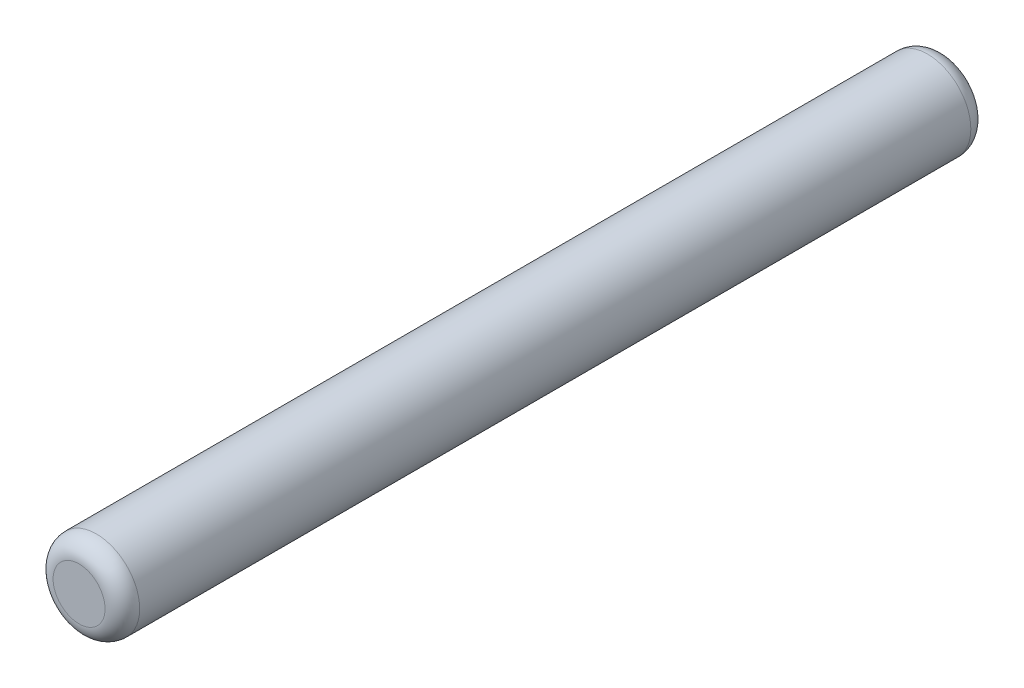
SolidWorks part; units mm, degrees
ref_plane "Front Plane" through (0, 0, 0) normal (0, 0, 1) x (1, 0, 0)
ref_plane "Top Plane" through (0, 0, 0) normal (0, 1, 0) x (1, 0, 0)
ref_plane "Right Plane" through (0, 0, 0) normal (1, 0, 0) x (0, 0, -1)
other "Configuration Table"
sketch "Sketch1" plane through (0, 0, 0) normal (0, 0, 1) x (1, 0, 0)
  circle A0 centre (0, 0) radius 0.75
  dimension "D1" = 1.5
extrude "Boss-Extrude1" add sketch "Sketch1" along normal blind 15
fillet "Fillet1" radius 0.3 2 edges at (0.75, 0, 0) (0.75, 0, 15)
